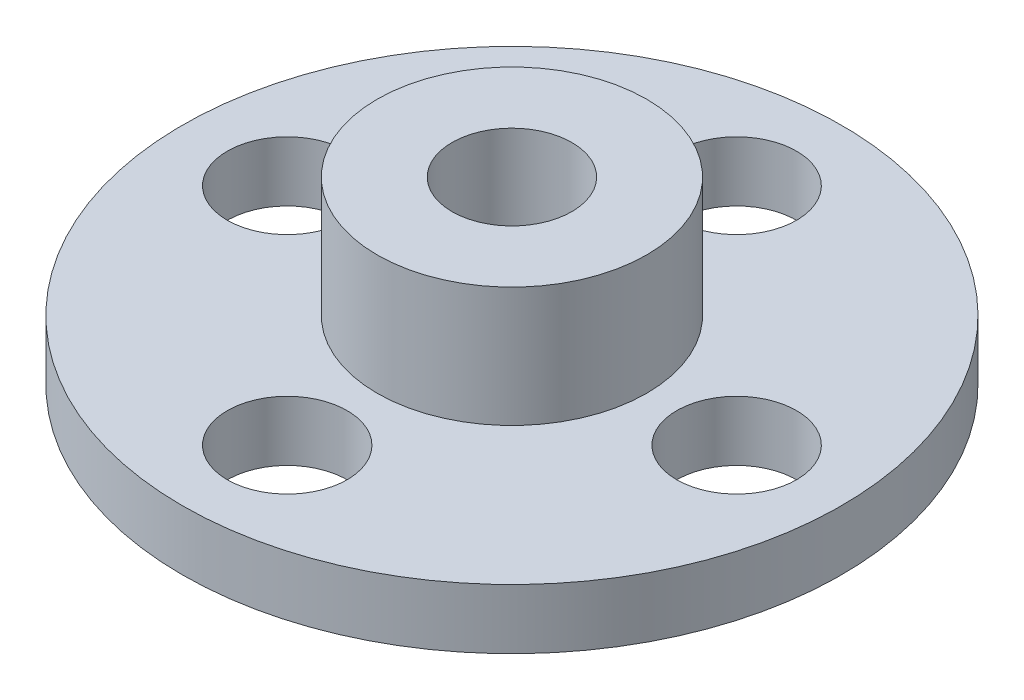
from build123d import *

# Parameters (mm, degrees)
SKETCH1_R               = 11
SKETCH1_R_2             = 2
BOSS_EXTRUDE1_DEPTH     = 2
SKETCH2_R               = 4.5
BOSS_EXTRUDE2_DEPTH     = 4
CUT_EXTRUDE1_DEPTH      = 17.673332001
CUT_EXTRUDE1_DEPTH_BACK = 17.673332001
SKETCH3_R               = 2


with BuildPart() as part:
    # Sketch1 → Boss-Extrude1 (new body)
    with BuildSketch(Plane(origin=(0, 0, 0), x_dir=(1, 0, 0), z_dir=(0, 1, 0))):
        with Locations(Location((0, 0, 0), (0, 0, 270))):
            Circle(SKETCH1_R)
        with Locations(Location((0, 7.5, 0), (0, 0, 270))):
            Circle(SKETCH1_R_2, mode=Mode.SUBTRACT)
        with Locations(Location((7.5, 0, 0), (0, 0, 270))):
            Circle(SKETCH1_R_2, mode=Mode.SUBTRACT)
        with Locations(Location((0, -7.5, 0), (0, 0, 270))):
            Circle(SKETCH1_R_2, mode=Mode.SUBTRACT)
        with Locations(Location((-7.5, 0, 0), (0, 0, 270))):
            Circle(SKETCH1_R_2, mode=Mode.SUBTRACT)
    extrude(amount=BOSS_EXTRUDE1_DEPTH)

    # Sketch2 → Boss-Extrude2 (add)
    with BuildSketch(Plane(origin=(0, 2, 0), x_dir=(1, 0, 0), z_dir=(0, 1, 0))):
        with Locations(Location((0, 0, 0), (0, 0, 270))):
            Circle(SKETCH2_R)
    extrude(amount=BOSS_EXTRUDE2_DEPTH)

    # Sketch3 → Cut-Extrude1 (cut, two sides: drawn at the far end of the back side and taken through both)
    with BuildSketch(Plane(origin=(0, 6, 0), x_dir=(1, 0, 0), z_dir=(0, 1, 0)).offset(-CUT_EXTRUDE1_DEPTH_BACK)):
        with Locations(Location((0, 0, 0), (0, 0, 270))):
            Circle(SKETCH3_R)
    extrude(amount=CUT_EXTRUDE1_DEPTH + CUT_EXTRUDE1_DEPTH_BACK, mode=Mode.SUBTRACT)


solid = part.part
